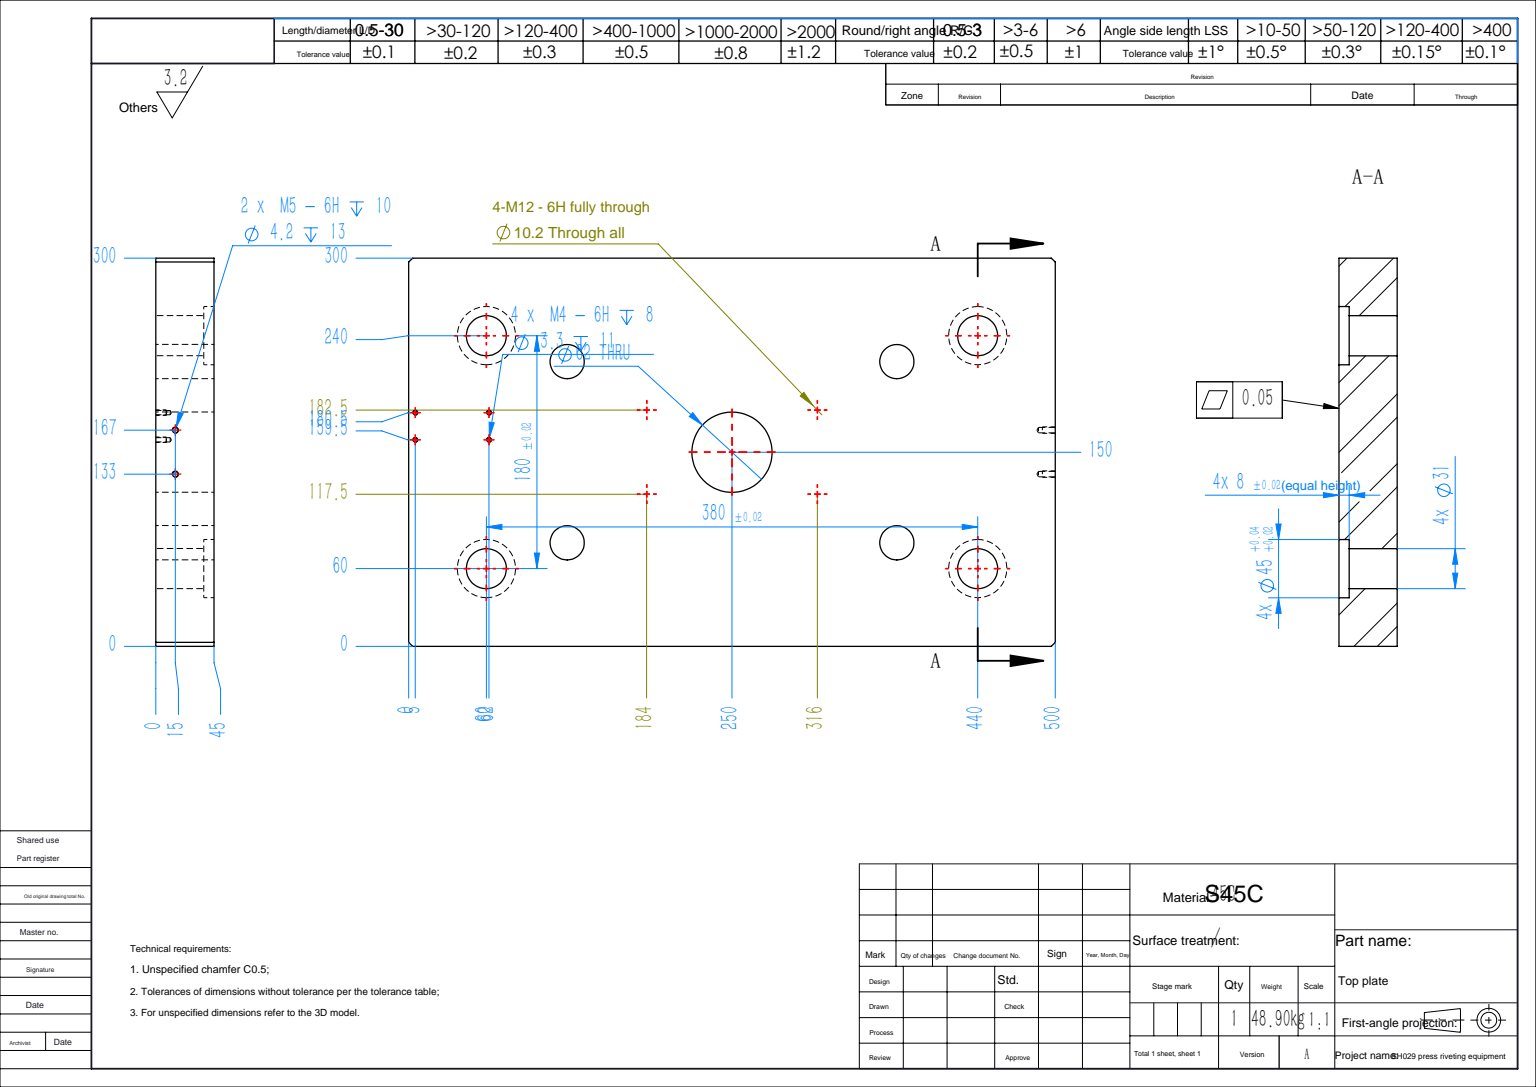
from build123d import *

# Parameters (mm, degrees)
SKETCH_1_W             = 500
SKETCH_1_H             = 300
EXTRUDE_1_DEPTH        = 45
SKETCH_2_R             = 22.5
CUT_EXTRUDE_1_DEPTH    = 8
CHAMFER_1_SIZE         = 3
SKETCH_16_R            = 15.5
CUT_EXTRUDE_3_DEPTH    = 296
SKETCH_17_R            = 31
CUT_EXTRUDE_4_DEPTH    = 296
HOLE_WIZARD_M4_1_D     = 3.3
HOLE_WIZARD_M4_1_DEPTH = 11
HOLE_WIZARD_M4_1_TIP   = 0.991420021
HOLE_WIZARD_M5_1_D     = 4.2
HOLE_WIZARD_M5_1_DEPTH = 13
HOLE_WIZARD_M5_1_TIP   = 1.2618073
HOLE_WIZARD_M30_1_D    = 26.5


with BuildPart() as part:
    # 草图1 → 凸台-拉伸1 (new body)
    with BuildSketch(Plane(origin=(0, 0, 0), x_dir=(1, 0, 0), z_dir=(0, 1, 0))):
        Rectangle(SKETCH_1_W, SKETCH_1_H)
    extrude(amount=EXTRUDE_1_DEPTH)

    # 草图2 → 切除-拉伸1 (cut)
    with BuildSketch(Plane.XZ):
        with Locations(Location((190, 90, 0), (0, 0, 270))):
            Circle(SKETCH_2_R)
        with Locations(Location((-190, 90, 0), (0, 0, 90))):
            Circle(SKETCH_2_R)
        with Locations(Location((190, -90, 0), (0, 0, 270))):
            Circle(SKETCH_2_R)
        with Locations(Location((-190, -90, 0), (0, 0, 90))):
            Circle(SKETCH_2_R)
    extrude(amount=-CUT_EXTRUDE_1_DEPTH, mode=Mode.SUBTRACT)

    # 倒角1
    chamfer_1_edges = [part.edges().sort_by_distance(p)[0] for p in [
        (250, 22.5, 150),
        (-250, 22.5, 150),
        (-250, 22.5, -150),
        (250, 22.5, -150),
    ]]
    chamfer(chamfer_1_edges, length=CHAMFER_1_SIZE)

    # 草图16 → 切除-拉伸3 (cut, through all)
    with BuildSketch(Plane(origin=(0, 45, 0), x_dir=(1, 0, 0), z_dir=(0, 1, 0))):
        with Locations(Location((190, -90, 0), (0, 0, 270))):
            Circle(SKETCH_16_R)
        with Locations(Location((190, 90, 0), (0, 0, 270))):
            Circle(SKETCH_16_R)
        with Locations(Location((-190, 90, 0), (0, 0, 270))):
            Circle(SKETCH_16_R)
        with Locations(Location((-190, -90, 0), (0, 0, 270))):
            Circle(SKETCH_16_R)
    extrude(amount=-CUT_EXTRUDE_3_DEPTH, mode=Mode.SUBTRACT)

    # 草图17 → 切除-拉伸4 (cut, through all)
    with BuildSketch(Plane.XZ):
        with Locations(Location((0, 0, 0), (0, 0, 270))):
            Circle(SKETCH_17_R)
    extrude(amount=-CUT_EXTRUDE_4_DEPTH, mode=Mode.SUBTRACT)

    # M4 螺纹孔1
    with Locations(Plane(origin=(0, 45, 0), x_dir=(1, 0, 0), z_dir=(0, 1, 0))):
        with Locations((-188, 30.5), (-245, 9.5), (-188, 9.5), (-245, 30.5)):
            Hole(HOLE_WIZARD_M4_1_D / 2, depth=HOLE_WIZARD_M4_1_DEPTH)
            with Locations((0, 0, -(HOLE_WIZARD_M4_1_DEPTH + HOLE_WIZARD_M4_1_TIP / 2))):  # 118° drill point
                Cone(0, HOLE_WIZARD_M4_1_D / 2, HOLE_WIZARD_M4_1_TIP, mode=Mode.SUBTRACT)

    # M5 螺纹孔1
    with Locations(Plane(origin=(250, 0, 0), x_dir=(0, 0, -1), z_dir=(1, 0, 0))):
        with Locations((-17, 30), (17, 30)):
            Hole(HOLE_WIZARD_M5_1_D / 2, depth=HOLE_WIZARD_M5_1_DEPTH)
            with Locations((0, 0, -(HOLE_WIZARD_M5_1_DEPTH + HOLE_WIZARD_M5_1_TIP / 2))):  # 118° drill point
                Cone(0, HOLE_WIZARD_M5_1_D / 2, HOLE_WIZARD_M5_1_TIP, mode=Mode.SUBTRACT)

    # M30 螺纹孔1 (through all)
    with Locations(Plane(origin=(0, 45, 0), x_dir=(1, 0, 0), z_dir=(0, 1, 0))):
        with Locations((-127.5, 70), (-127.5, -70), (127.5, 70), (127.5, -70)):
            Hole(HOLE_WIZARD_M30_1_D / 2)


solid = part.part
